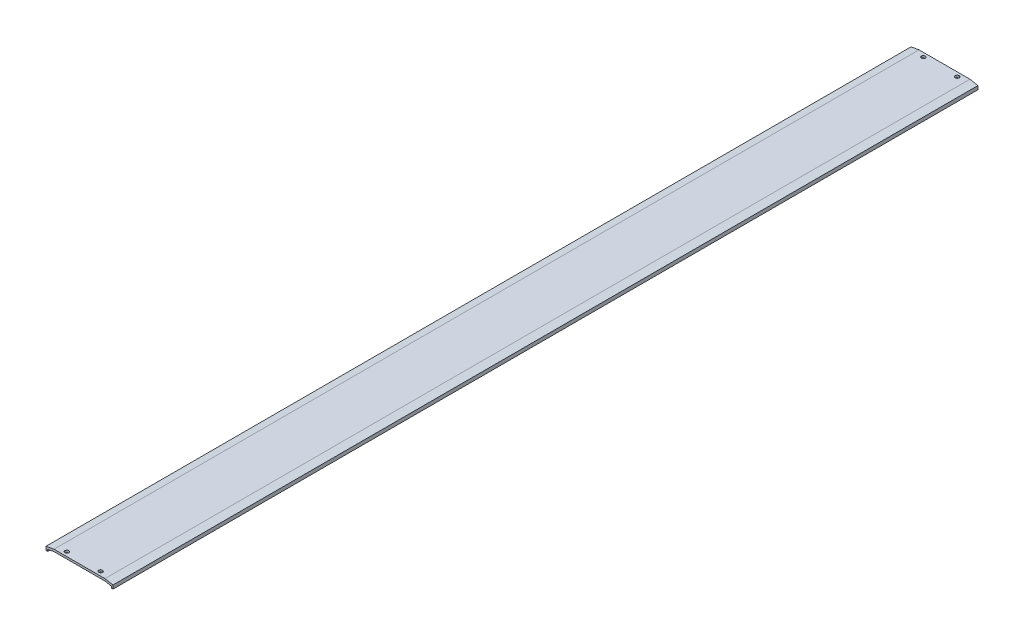
from build123d import *

# Parameters (mm, degrees)
EXTRUDE_1_DEPTH     = 510
SKETCH_2_R          = 2.25
CUT_EXTRUDE_1_DEPTH = 20


with BuildPart() as part:
    # 草图1 → 凸台-拉伸1 (new, symmetric)
    with BuildSketch(Plane.XY):
        Polygon((-37.5, 0), (-39.5, 0), (-39.5, 4.3), (-30, 6), (30, 6), (39.5, 4.3), (39.5, 0), (37.5, 0), (37.5, 2.122105263), (29.8, 3.5), (-29.8, 3.5), (-37.5, 2.122105263), align=None)
    extrude(amount=EXTRUDE_1_DEPTH, both=True)

    # 草图2 → 切除-拉伸1 (cut)
    with BuildSketch(Plane(origin=(0, 6, 0), x_dir=(1, 0, 0), z_dir=(0, 1, 0))):
        with Locations(Location((-20, 505, 0), (0, 0, 270))):
            Circle(SKETCH_2_R)
        with Locations(Location((20, 505, 0), (0, 0, 270))):
            Circle(SKETCH_2_R)
    cut_extrude_1 = extrude(amount=-CUT_EXTRUDE_1_DEPTH, mode=Mode.SUBTRACT)

    # 镜向1: 切除-拉伸1 across plane
    add(cut_extrude_1.mirror(Plane.XY), mode=Mode.SUBTRACT)


solid = part.part
